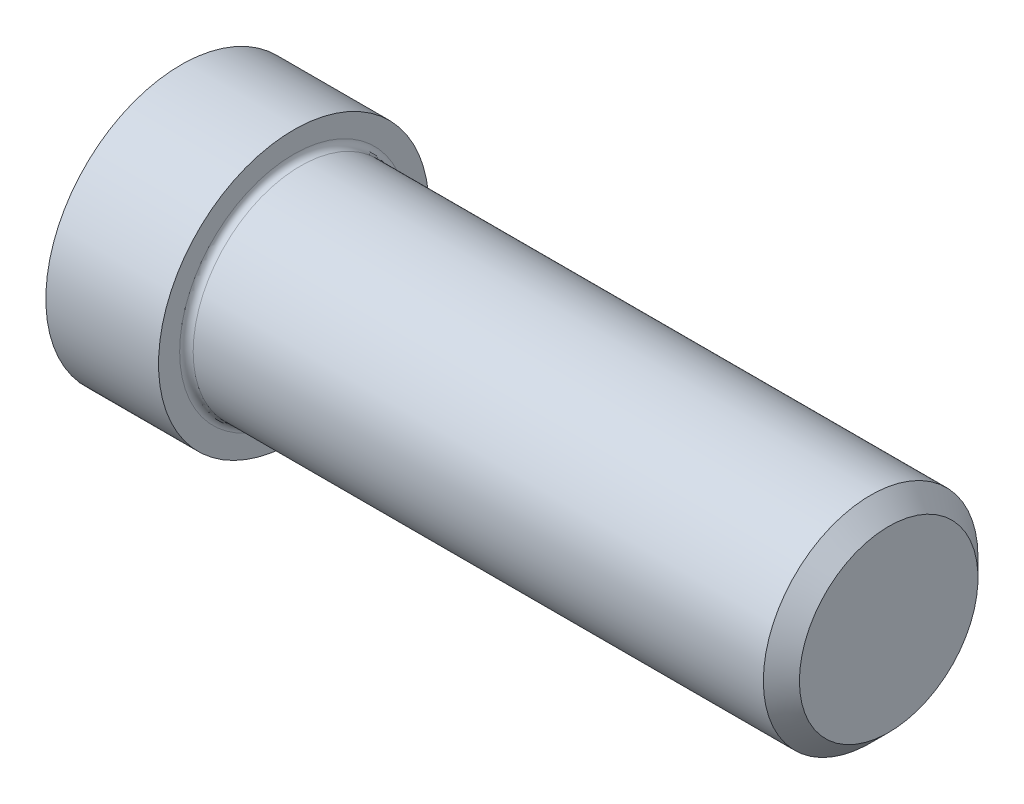
from build123d import *

# Parameters (mm, degrees)
SKETCH1_R          = 12
BASE_EXTRUDE_DEPTH = 10
CHAMFER_2_SIZE     = 1.6
FILLET_2_R         = 0.6
CUT_EXTRUDE1_DEPTH = 7.62


with BuildPart() as part:
    # Sketch1 → Base-Extrude (new body)
    with BuildSketch(Plane(origin=(0, 0, 0), x_dir=(0, 0, -1), z_dir=(1, 0, 0))):
        Circle(SKETCH1_R)
    extrude(amount=BASE_EXTRUDE_DEPTH)

    # Sketch2 → Boss-Revolve1 (revolve)
    with BuildSketch(Plane.XY, mode=Mode.PRIVATE) as boss_revolve1_sk:
        Polygon((0, 0), (62.8, 0), (62.8, 6.268), (62.8, 9.525), (27.8072, 9.525), (0, 9.525), align=None)
    revolve(boss_revolve1_sk.sketch.rotate(Axis((0, 0, 0), (1, 0, 0)), 90), axis=Axis((0, 0, 0), (1, 0, 0)))

    # Chamfer 2
    chamfer_2_edges = [part.edges().sort_by_distance(p)[0] for p in [
        (62.8, 0, -9.525),
    ]]
    chamfer(chamfer_2_edges, length=CHAMFER_2_SIZE)

    # Fillet 2
    fillet_2_edges = [part.edges().sort_by_distance(p)[0] for p in [
        (10, 0, -9.525),
    ]]
    fillet(fillet_2_edges, radius=FILLET_2_R)

    # Sketch7 → Cut-Extrude1 (cut)
    with BuildSketch(Plane.ZY):
        Polygon((-8.76789552, 5.062146839), (-8.76789552, -5.062146839), (0, -10.124293677), (8.76789552, -5.062146839), (8.76789552, 5.062146839), (0, 10.124293677), align=None)
    extrude(amount=-CUT_EXTRUDE1_DEPTH, mode=Mode.SUBTRACT)


solid = part.part
